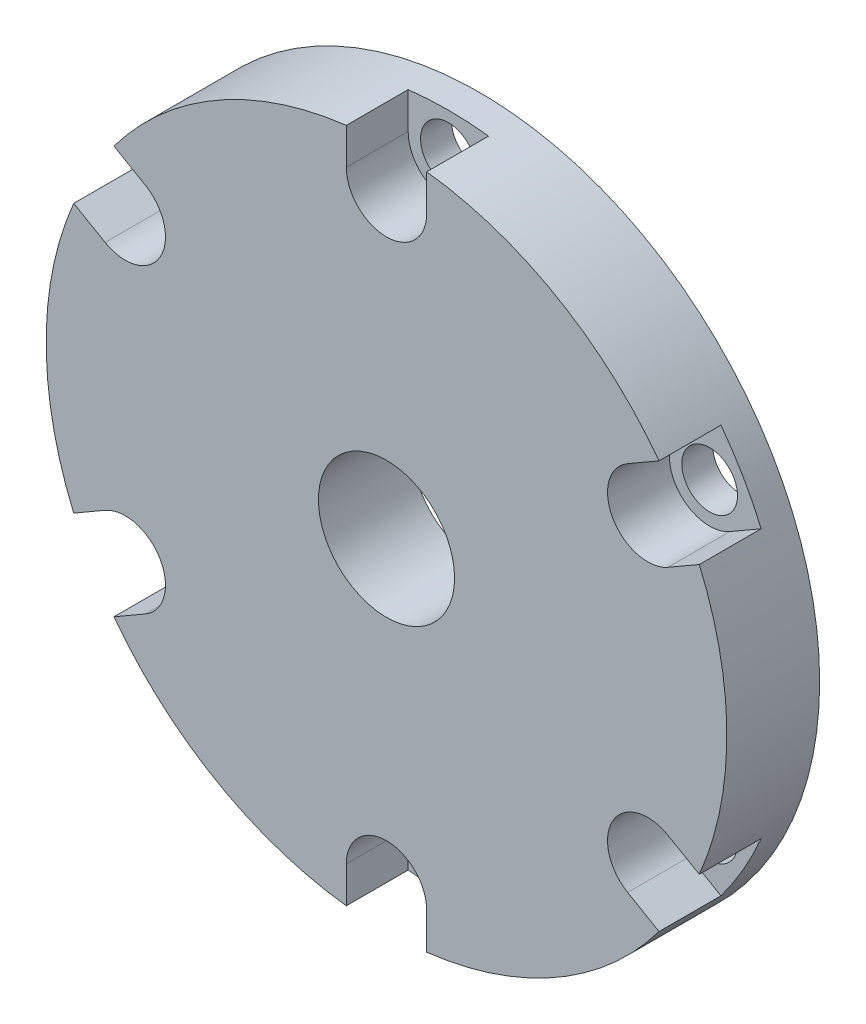
SolidWorks part; units mm, degrees
ref_plane "Front Plane" through (0, 0, 0) normal (0, 0, 1) x (1, 0, 0)
ref_plane "Top Plane" through (0, 0, 0) normal (0, 1, 0) x (1, 0, 0)
ref_plane "Right Plane" through (0, 0, 0) normal (1, 0, 0) x (0, 0, -1)
sketch "Sketch1" plane through (0, 0, 0) normal (0, 0, 1) x (1, 0, 0)
  circle A0 centre (0, 0) radius 110
  circle A1 centre (0, 0) radius 97.5 construction
  circle A2 centre (0, 97.5) radius 9
  circle A3 centre (84.4375, 48.75) radius 9
  circle A4 centre (84.4375, -48.75) radius 9
  circle A5 centre (0, -97.5) radius 9
  circle A6 centre (-84.4375, -48.75) radius 9
  circle A7 centre (-84.4375, 48.75) radius 9
  circle A8 centre (0, 0) radius 22
  point P19 (0, 0)
  dimension "D1" = 220
  dimension "D2" = 195
  dimension "D3" = 18
  dimension "D4" = 44
extrude "Boss-Extrude1" add sketch "Sketch1" along normal blind 30
sketch "Sketch2" plane through (0, 0, 30) normal (0, 0, 1) x (1, 0, 0)
  line L0 (-13, 97.5) -> (-13, 114.5314)
  line L1 (-13, 114.5314) -> (13, 114.5314)
  line L2 (13, 114.5314) -> (13, 97.5)
  line L3 (105.6871, 46.0074) -> (90.9375, 37.4917)
  line L4 (92.6871, 68.5241) -> (105.6871, 46.0074)
  line L5 (77.9375, 60.0083) -> (92.6871, 68.5241)
  line L6 (92.6871, -68.5241) -> (77.9375, -60.0083)
  line L7 (105.6871, -46.0074) -> (92.6871, -68.5241)
  line L8 (90.9375, -37.4917) -> (105.6871, -46.0074)
  line L9 (-13, -114.5314) -> (-13, -97.5)
  line L10 (13, -114.5314) -> (-13, -114.5314)
  line L11 (13, -97.5) -> (13, -114.5314)
  line L12 (-105.6871, -46.0074) -> (-90.9375, -37.4917)
  line L13 (-92.6871, -68.5241) -> (-105.6871, -46.0074)
  line L14 (-77.9375, -60.0083) -> (-92.6871, -68.5241)
  line L15 (-92.6871, 68.5241) -> (-77.9375, 60.0083)
  line L16 (-105.6871, 46.0074) -> (-92.6871, 68.5241)
  line L17 (-90.9375, 37.4917) -> (-105.6871, 46.0074)
  arc A0 (-13, 97.5) -> (13, 97.5) centre (0, 97.5) ccw
  arc A1 (77.9375, 60.0083) -> (90.9375, 37.4917) centre (84.4375, 48.75) ccw
  arc A2 (90.9375, -37.4917) -> (77.9375, -60.0083) centre (84.4375, -48.75) ccw
  arc A3 (13, -97.5) -> (-13, -97.5) centre (0, -97.5) ccw
  arc A4 (-77.9375, -60.0083) -> (-90.9375, -37.4917) centre (-84.4375, -48.75) ccw
  arc A5 (-90.9375, 37.4917) -> (-77.9375, 60.0083) centre (-84.4375, 48.75) ccw
  point P34 (0, 0)
  dimension "D1" = 26
extrude "Cut-Extrude1" cut sketch "Sketch2" against normal blind 20
